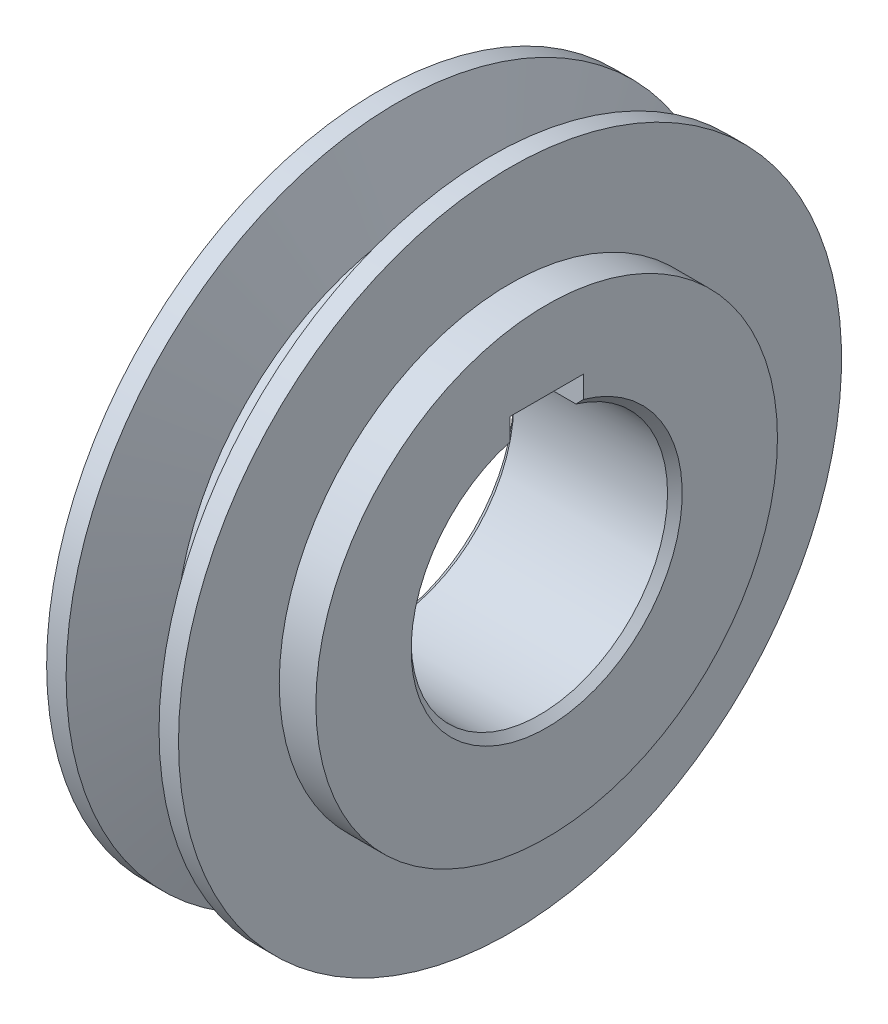
from build123d import *

# Parameters (mm, degrees)
CHAMFER_1_SIZE      = 1
SKETCH_4_W          = 10
SKETCH_4_H          = 4.029490121
CUT_EXTRUDE_1_DEPTH = 69.000919111


with BuildPart() as part:
    # 草图1 → 旋转1 (revolve)
    with BuildSketch(Plane.XY, mode=Mode.PRIVATE) as revolve_1_sk:
        Polygon((0, 17.5), (0, 45.25), (18, 45.25), (18, 31.5), (23, 31.5), (23, 17.5), align=None)
    revolve(revolve_1_sk.sketch.rotate(Axis((0, 0, 0), (1, 0, 0)), 90), axis=Axis((0, 0, 0), (1, 0, 0)))

    # 草图2 → 切除-旋转1 (revolve, cut)
    with BuildSketch(Plane.XY, mode=Mode.PRIVATE) as cut_revolve_1_sk:
        Polygon((11.840143071, 33.8), (15.340759374, 45.25), (2.659240626, 45.25), (6.159856929, 33.8), align=None)
    revolve(cut_revolve_1_sk.sketch.rotate(Axis((0, 0, 0), (1, 0, 0)), 90), axis=Axis((0, 0, 0), (1, 0, 0)), mode=Mode.SUBTRACT)

    # 倒角1
    chamfer_1_edges = [part.edges().sort_by_distance(p)[0] for p in [
        (0, 0, -17.5),
        (23, 0, -17.5),
    ]]
    chamfer(chamfer_1_edges, length=CHAMFER_1_SIZE)

    # 草图4 → 切除-拉伸1 (cut, through all)
    with BuildSketch(Plane.ZY):
        with Locations((0, 18.785254892)):
            Rectangle(SKETCH_4_W, SKETCH_4_H)
    extrude(amount=-CUT_EXTRUDE_1_DEPTH, mode=Mode.SUBTRACT)


solid = part.part
